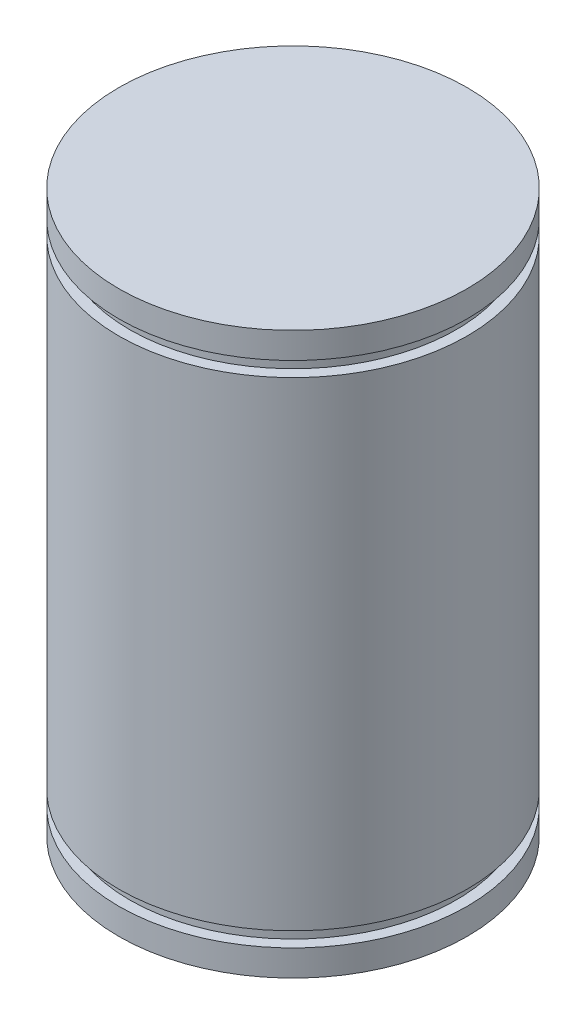
SolidWorks part; units mm, degrees
material "合金钢"
ref_plane "前视基准面" through (0, 0, 0) normal (0, 0, 1) x (1, 0, 0)
ref_plane "上视基准面" through (0, 0, 0) normal (0, 1, 0) x (1, 0, 0)
ref_plane "右视基准面" through (0, 0, 0) normal (1, 0, 0) x (0, 0, -1)
sketch "草图1" plane through (0, 0, 0) normal (0, 1, 0) x (1, 0, 0)
  circle A0 centre (0, 0) radius 20
  dimension "D1" = 40
extrude "凸台-拉伸1" add sketch "草图1" along normal blind 64.4
sketch "草图2" plane through (0, 0, 0) normal (0, 0, 1) x (1, 0, 0)
  line L0 (20, 64.4) -> (-20, 64.4) construction
  line L1 (-22.0759, 61.4) -> (-18.75, 61.4)
  line L2 (-22.0759, 61.4) -> (-22.0759, 59.7)
  line L3 (-22.0759, 59.7) -> (-18.75, 59.7)
  line L4 (-18.75, 61.4) -> (-18.75, 59.7)
  dimension "D1" = 3
  dimension "D2" = 1.7
  dimension "D3" = 18.75
revolve "切除-旋转1" cut sketch "草图2" angle 360 about axis through (0, 64.4, 0) along (0, -1, 0)
ref_plane "基准面1" through (0, 32.2, 0) normal (0, -1, 0) x (-1, 0, 0)
mirror "镜向1" about plane through (0, 32.2, 0) normal (0, -1, 0) of "切除-旋转1"
